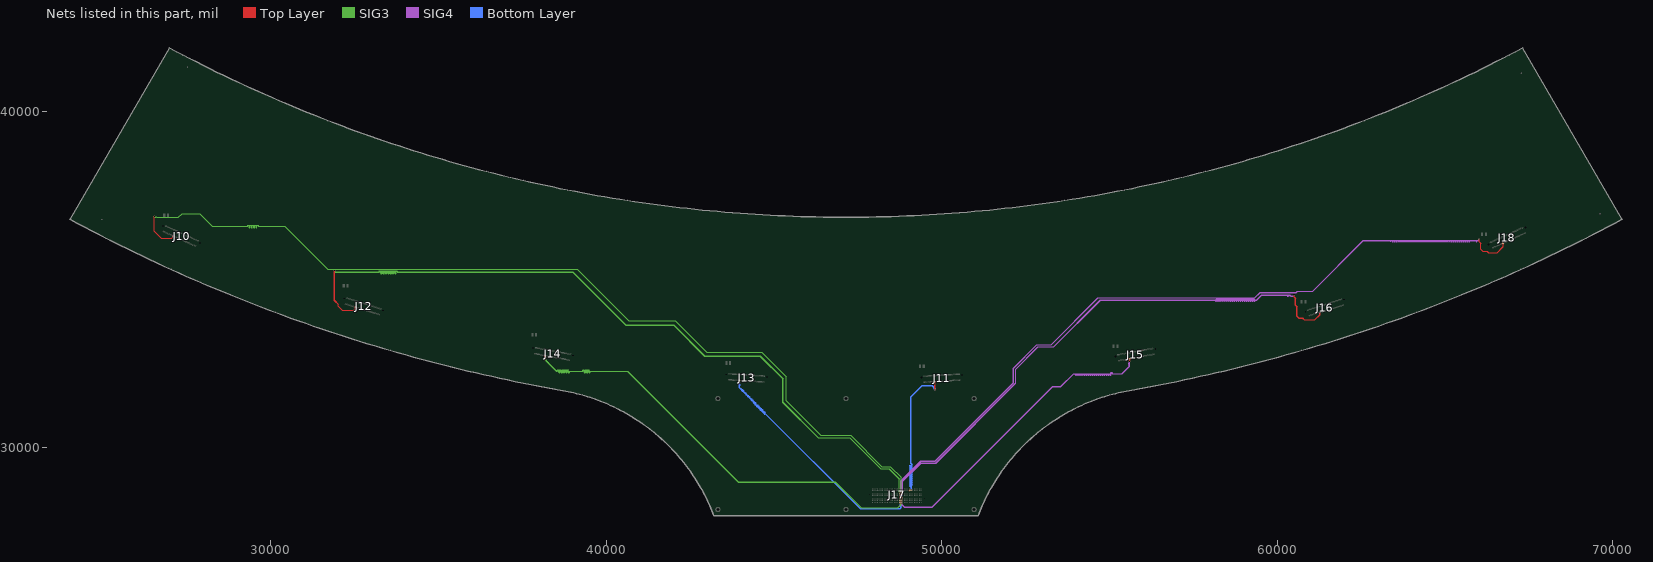
[diagram p0: the nets of this part, all layers, seen from the top]
# Altium PCB MISC86329.PcbDoc (part 5 of 11)
Units mil, origin at the board's own origin, x right, y up, seen from the top; angles counter-clockwise.
Board outline 46247.15 x 13937.21 mil, 6 copper layers (Top Layer, GND2, SIG3, SIG4, POWER5, Bottom Layer); 17 components, 210 nets, 908 pads, 1109 vias.

## Via types
v1: diameter 24, hole 12, Top Layer to Bottom Layer, 684 vias
v2: diameter 18, hole 9, Top Layer to Bottom Layer, 425 vias

## Nets (pads, with @x,y where several pads share a name; then routed paths per layer and width w, separated by ;. In a path a pad name is that pad's centre, name@x,y a point inside that pad or via, vN(x,y) a via of type N, cw(c..) or ccw(c..) an arc to the next point about the centre after c; other vN are vias at no path point) (continued)
DATAIN3N_CH1: J12.23 J17.F14 | length 23101.3
  Top Layer w5: v2(31893.5,35275) 31900,35268.5 31900,34381.86 32013,34268.86 32013,34213.86 32139.86,34087 32489.14,34087 32533.06,34130.92 32533.06,34159.09 J12.23@32553.09,34179.11 ; J17.F14@48737.89,28618.8 v2(48761.69,28642.61)
  SIG3 w5: v2(31893.5,35275) 31900,35268.5 31900,35252.86 31921.43,35231.43 ; 31920,35233 31929,35224 32003,35224 ; 31986.86,35224 32003,35224 ; v2(48761.69,28642.61) 48759.39,28642.61 48749.96,28652.04 48732,28670 48732,29060 48428,29364 48181.86,29364 47259.86,30286 46320.86,30286 45264,31342.86 45264,32047 44583,32728 42928.86,32728 42011.86,33645 40582.86,33645 39003.86,35224 33783.18,35224 33771.5,35235.68 33771.5,35257.84 33765.68,35263.67 33752.32,35263.67 33746.5,35257.84 33746.5,35196.01 33734.82,35184.33 33713.18,35184.33 33701.5,35196.01 33701.5,35257.84 33695.68,35263.67 33682.32,35263.67 33676.5,35257.84 33676.5,35196.01 33664.82,35184.33 33643.18,35184.33 33631.5,35196.01 33631.5,35257.84 33625.68,35263.67 33612.32,35263.67 33606.5,35257.84 33606.5,35196.01 33594.82,35184.33 33573.18,35184.33 33561.5,35196.01 33561.5,35257.84 33555.68,35263.67 33542.32,35263.67 33536.5,35257.84 33536.5,35196.01 33524.82,35184.33 33503.18,35184.33 33491.5,35196.01 33491.5,35257.84 33485.68,35263.67 33472.32,35263.67 33466.5,35257.84 33466.5,35196.01 33454.82,35184.33 33433.18,35184.33 33421.5,35196.01 33421.5,35257.84 33415.68,35263.67 33402.32,35263.67 33396.5,35257.84 33396.5,35196.01 33384.82,35184.33 33363.18,35184.33 33351.5,35196.01 33351.5,35257.84 33345.68,35263.67 33332.32,35263.67 33326.5,35257.84 33326.5,35196.01 33314.82,35184.33 33293.18,35184.33 33281.5,35196.01 33281.5,35257.84 33275.68,35263.67 33262.32,35263.67 33256.5,35257.84 33256.5,35235.68 33244.82,35224 32003,35224
DATAIN3N_CH2: J14.23 J17.B14 | length 13805.7
  Top Layer w5: v2(38195.5,32680) 38189,32686.5 38189,32711 38200,32722 J14.23@38200,32734 ; J17.B14@48737.89,28418.8 v2(48761.69,28395)
  SIG3 w5: v2@38194,32677 38188,32671 38188,32618 38192.42,32613.58 38201.26,32613.58 38202.28,32614.6 38211.11,32614.6 38219.95,32605.76 38219.95,32596.92 38218.94,32595.9 38218.94,32587.06 38227.77,32578.23 38236.61,32578.23 38237.56,32579.18 38246.4,32579.18 38255.24,32570.34 38255.24,32561.5 38254.29,32560.55 38254.29,32551.71 38263.13,32542.87 38271.97,32542.87 38272.92,32543.82 38281.76,32543.82 38290.6,32534.98 38290.6,32526.14 38289.65,32525.19 38289.65,32516.35 38526,32280 38546.68,32280 38552.5,32285.82 38552.5,32308.32 38564.18,32320 38585.82,32320 38597.5,32308.32 38597.5,32245.82 38603.32,32240 38616.68,32240 38622.5,32245.82 38622.5,32308.32 38634.18,32320 38655.82,32320 38667.5,32308.32 38667.5,32245.82 38673.32,32240 38686.68,32240 38692.5,32245.82 38692.5,32308.32 38704.18,32320 38725.82,32320 38737.5,32308.32 38737.5,32245.82 38743.32,32240 38756.68,32240 38762.5,32245.82 38762.5,32308.32 38774.18,32320 38795.82,32320 38807.5,32308.32 38807.5,32245.82 38813.32,32240 38826.68,32240 38832.5,32245.82 38832.5,32308.32 38844.18,32320 38865.82,32320 38877.5,32308.32 38877.5,32245.82 38883.32,32240 38896.68,32240 38902.5,32245.82 38902.5,32268.32 38914.18,32280 39302.68,32280 39308.5,32285.82 39308.5,32304.42 39320.18,32316.1 39341.82,32316.1 39353.5,32304.42 39353.5,32249.72 39359.32,32243.9 39372.68,32243.9 39378.5,32249.72 39378.5,32304.42 39390.18,32316.1 39411.82,32316.1 39423.5,32304.42 39423.5,32249.72 39429.32,32243.9 39442.68,32243.9 39448.5,32249.72 39448.5,32304.42 39460.18,32316.1 39481.82,32316.1 39493.5,32304.42 39493.5,32249.72 39499.32,32243.9 39512.68,32243.9 39518.5,32249.72 39518.5,32268.32 39530.18,32280 40641,32280 43937,28984 46829,28984 47603,28210 48693.69,28210 48781.69,28298 48781.69,28375 v2(48761.69,28395)
DATAIN3N_CH3: J13.23 J17.A14 | length 7749.3
  Top Layer w5: 43978.23,31941.5 43978.23,31959.28 43988.94,31970 J13.23@43988.94,31998.95 ; J17.A14@48737.89,28368.8 v2(48761.69,28345)
  Bottom Layer w5: v2(43984.73,31935) 43984.73,31934.67 43978,31927.94 43978,31893.5 43983,31888.5 43996.72,31888.5 44001.72,31883.5 44001.72,31868.5 43996.72,31863.5 43983,31863.5 43978,31858.5 43978,31783.14 43995.03,31766.12 43999.72,31766.12 44005.03,31771.42 44018.01,31771.42 44029.77,31759.65 44029.77,31746.67 44024.47,31741.37 44024.47,31736.67 44030.38,31730.76 44035.08,31730.76 44040.38,31736.06 44053.36,31736.06 44065.13,31724.3 44065.13,31711.32 44059.83,31706.01 44059.83,31701.32 44065.74,31695.41 44070.43,31695.41 44075.74,31700.71 44088.72,31700.71 44100.49,31688.94 44100.49,31675.96 44095.18,31670.66 44095.18,31665.96 44101.09,31660.05 44105.79,31660.05 44111.09,31665.35 44124.07,31665.35 44135.84,31653.59 44135.84,31640.6 44130.54,31635.3 44130.54,31630.6 44136.45,31624.69 44141.14,31624.69 44146.45,31630 44159.43,31630 44171.2,31618.23 44171.2,31605.25 44165.89,31599.95 44165.89,31595.25 44171.8,31589.34 44176.5,31589.34 44181.8,31594.64 44194.78,31594.64 44206.55,31582.88 44206.55,31569.89 44201.25,31564.59 44201.25,31559.89 44207.16,31553.98 44211.85,31553.98 44217.16,31559.29 44230.14,31559.29 44241.91,31547.52 44241.91,31534.54 44236.6,31529.24 44236.6,31524.54 44242.51,31518.63 44247.21,31518.63 44252.51,31523.93 44265.49,31523.93 44277.26,31512.16 44277.26,31499.18 44271.96,31493.88 44271.96,31489.18 44277.87,31483.27 44282.57,31483.27 44287.87,31488.58 44300.85,31488.58 44312.62,31476.81 44312.62,31463.83 44307.31,31458.52 44307.31,31453.83 44313.22,31447.92 44317.92,31447.92 44323.22,31453.22 44336.2,31453.22 44347.97,31441.45 44347.97,31428.47 44342.67,31423.17 44342.67,31418.47 44348.58,31412.56 44353.28,31412.56 44358.58,31417.87 44371.56,31417.87 44383.33,31406.1 44383.33,31393.12 44378.02,31387.81 44378.02,31383.12 44383.93,31377.21 44388.63,31377.21 44393.93,31382.51 44406.92,31382.51 44418.68,31370.74 44418.68,31357.76 44399.24,31338.32 44399.24,31333.62 44405.15,31327.71 44409.84,31327.71 44429.29,31347.16 44442.27,31347.16 44454.04,31335.39 44454.04,31322.41 44434.59,31302.96 44434.59,31298.26 44440.5,31292.35 44445.2,31292.35 44464.65,31311.8 44477.63,31311.8 44489.39,31300.03 44489.39,31287.05 44469.95,31267.61 44469.95,31262.91 44475.86,31257 44480.56,31257 44500,31276.44 44512.98,31276.44 44524.75,31264.68 44524.75,31251.7 44505.3,31232.25 44505.3,31227.55 44511.21,31221.64 44515.91,31221.64 44535.36,31241.09 44548.34,31241.09 44560.1,31229.32 44560.1,31216.34 44540.66,31196.9 44540.66,31192.2 44546.57,31186.29 44551.27,31186.29 44570.71,31205.73 44583.69,31205.73 44595.46,31193.97 44595.46,31180.99 44576.01,31161.54 44576.01,31156.84 44581.92,31150.93 44586.62,31150.93 44606.07,31170.38 44619.05,31170.38 44630.82,31158.61 44630.82,31145.63 44611.37,31126.18 44611.37,31121.49 44617.28,31115.58 44621.98,31115.58 44641.42,31135.02 44654.4,31135.02 44666.17,31123.26 44666.17,31110.27 44646.73,31090.83 44646.73,31086.13 44652.64,31080.22 44657.33,31080.22 44676.78,31099.67 44689.76,31099.67 44701.53,31087.9 44701.53,31074.92 44682.08,31055.47 44682.08,31050.78 44687.99,31044.87 44692.69,31044.87 44712.13,31064.31 44725.11,31064.31 44736.88,31052.54 44736.88,31039.56 44717.44,31020.12 44717.44,31015.42 44723.35,31009.51 44728.04,31009.51 44731.53,31013 44748.14,31013 47576.14,28185 48759,28185 48781.69,28207.69 48781.69,28223.18 48778.37,28226.5 48770.87,28226.5 48761.69,28235.68 48761.69,28252.32 48770.87,28261.5 48798.37,28261.5 48801.69,28264.82 48801.69,28273.18 48798.37,28276.5 48770.87,28276.5 48761.69,28285.68 48761.69,28302.32 48770.87,28311.5 48778.37,28311.5 48781.69,28314.82 48781.69,28325 v2(48761.69,28345)
DATAIN3N_CH4: J11.23 J17.H8 | length 5094.4
  Top Layer w5: J17.H8@49037.89,28718.8 v2(49061.69,28742.61) ; 49809.93,31719.5 49809.93,31933.28 49820.65,31944 J11.23@49820.65,31969.08
  Bottom Layer w5: v2(49061.69,28742.61) 49081.69,28762.61 49081.69,28831.93 49075.62,28838 49063.62,28838 49051.69,28849.93 49051.69,28866.07 49063.62,28878 49105.62,28878 49111.69,28884.07 49111.69,28891.93 49105.62,28898 49063.62,28898 49051.69,28909.93 49051.69,28926.07 49063.62,28938 49105.62,28938 49111.69,28944.07 49111.69,28951.93 49105.62,28958 49063.62,28958 49051.69,28969.93 49051.69,28986.07 49063.62,28998 49105.62,28998 49111.69,29004.07 49111.69,29011.93 49105.62,29018 49063.62,29018 49051.69,29029.93 49051.69,29046.07 49063.62,29058 49105.62,29058 49111.69,29064.07 49111.69,29071.93 49105.62,29078 49063.62,29078 49051.69,29089.93 49051.69,29106.07 49063.62,29118 49105.62,29118 49111.69,29124.07 49111.69,29131.93 49105.62,29138 49063.62,29138 49051.69,29149.93 49051.69,29166.07 49063.62,29178 49105.62,29178 49111.69,29184.07 49111.69,29191.93 49105.62,29198 49063.62,29198 49051.69,29209.93 49051.69,29226.07 49063.62,29238 49105.62,29238 49111.69,29244.07 49111.69,29251.93 49105.62,29258 49063.62,29258 49051.69,29269.93 49051.69,29286.07 49063.62,29298 49105.62,29298 49111.69,29304.07 49111.69,29311.93 49105.62,29318 49063.62,29318 49051.69,29329.93 49051.69,29346.07 49063.62,29358 49105.62,29358 49111.69,29364.07 49111.69,29371.93 49105.62,29378 49063.62,29378 49051.69,29389.93 49051.69,29406.07 49063.62,29418 49105.62,29418 49111.69,29424.07 49111.69,29431.93 49105.62,29438 49063.62,29438 49051.69,29449.93 49051.69,29466.07 49063.62,29478 49101.86,29478 49108,29484.14 49108,29496 49081.69,29522.31 49081.69,31519.69 49421,31859 49712.14,31859 49810,31761.14 49810,31720 v2@49814,31716
  other v2: 49816.43,31713
DATAIN3N_CH5: J15.23 J17.C14 | length 10126
  Top Layer w5: J17.C14@48737.89,28468.8 v2(48761.69,28445) ; v2(55610.5,32567) 55604,32573.5 55604,32615.47 55612.53,32624 J15.23@55612.53,32650.14
  SIG4 w5: v2(48761.69,28445) 48781.69,28425 48781.69,28323.17 48878.86,28226 49724.14,28226 53312.14,31814 53553,31814 53936,32197 53981.43,32197 53986,32192.43 53986,32169.16 53996.43,32158.73 54015.57,32158.73 54026,32169.16 54026,32192.43 54030.57,32197 54041.43,32197 54046,32192.43 54046,32169.16 54056.43,32158.73 54075.57,32158.73 54086,32169.16 54086,32192.43 54090.57,32197 54101.43,32197 54106,32192.43 54106,32169.16 54116.43,32158.73 54135.57,32158.73 54146,32169.16 54146,32192.43 54150.57,32197 54161.43,32197 54166,32192.43 54166,32169.16 54176.43,32158.73 54195.57,32158.73 54206,32169.16 54206,32192.43 54210.57,32197 54221.43,32197 54226,32192.43 54226,32169.16 54236.43,32158.73 54255.57,32158.73 54266,32169.16 54266,32192.43 54270.57,32197 54281.43,32197 54286,32192.43 54286,32169.16 54296.43,32158.73 54315.57,32158.73 54326,32169.16 54326,32192.43 54330.57,32197 54341.43,32197 54346,32192.43 54346,32169.16 54356.43,32158.73 54375.57,32158.73 54386,32169.16 54386,32192.43 54390.57,32197 54401.43,32197 54406,32192.43 54406,32169.16 54416.43,32158.73 54435.57,32158.73 54446,32169.16 54446,32192.43 54450.57,32197 54461.43,32197 54466,32192.43 54466,32169.16 54476.43,32158.73 54495.57,32158.73 54506,32169.16 54506,32192.43 54510.57,32197 54521.43,32197 54526,32192.43 54526,32169.16 54536.43,32158.73 54555.57,32158.73 54566,32169.16 54566,32192.43 54570.57,32197 54581.43,32197 54586,32192.43 54586,32169.16 54596.43,32158.73 54615.57,32158.73 54626,32169.16 54626,32192.43 54630.57,32197 54641.43,32197 54646,32192.43 54646,32169.16 54656.43,32158.73 54675.57,32158.73 54686,32169.16 54686,32192.43 54690.57,32197 54701.43,32197 54706,32192.43 54706,32169.16 54716.43,32158.73 54735.57,32158.73 54746,32169.16 54746,32192.43 54750.57,32197 54761.43,32197 54766,32192.43 54766,32169.16 54776.43,32158.73 54795.57,32158.73 54806,32169.16 54806,32192.43 54810.57,32197 54821.43,32197 54826,32192.43 54826,32169.16 54836.43,32158.73 54855.57,32158.73 54866,32169.16 54866,32192.43 54870.57,32197 54881.43,32197 54886,32192.43 54886,32169.16 54896.43,32158.73 54915.57,32158.73 54926,32169.16 54926,32192.43 54930.57,32197 54941.43,32197 54946,32192.43 54946,32169.16 54956.43,32158.73 54975.57,32158.73 54986,32169.16 54986,32192.43 54990.57,32197 55001.43,32197 55006,32192.43 55006,32169.16 55016.43,32158.73 55035.57,32158.73 55046,32169.16 55046,32230.69 55050.57,32235.27 55061.43,32235.27 55066,32230.69 55066,32207.43 55076.43,32197 55377,32197 55604,32424 55604,32441 55604,32447 55604,32477 55604,32487 55604,32517 55604,32532 55604,32542 55604,32558 v2@55610,32564
DATAIN3N_CH6: J16.23 J17.D14 | length 18293.9
  Top Layer w5: J17.D14@48737.89,28518.8 v2(48761.69,28495) ; v2(60484.5,34554) 60491,34547.5 60491,34491 60535,34447 60535,34235 60581,34189 60581,33910.86 60635.86,33856 60747.86,33856 60800.86,33803 61119.14,33803 61277,33960.86 61277,34003.76 61278.24,34005 J16.23@61278.24,34031.97
  SIG4 w5: v2(48761.69,28495) 48788.36,28495 48804.86,28511.5 48814.05,28511.5 48830,28527.45 48830,28997.14 49382.86,29550 49827,29550 52202,31925 52202,32341.14 52867.86,33007 53336,33007 54730,34401 58144,34401 58167.93,34377.07 58168,34377.07 58172.07,34373 58181.86,34373 58188,34379.14 58188,34419.07 58199.93,34431 58216.07,34431 58228,34419.07 58228,34377.07 58234.07,34371 58241.93,34371 58248,34377.07 58248,34419.07 58259.93,34431 58276.07,34431 58288,34419.07 58288,34377.07 58294.07,34371 58301.93,34371 58308,34377.07 58308,34419.07 58319.93,34431 58336.07,34431 58348,34419.07 58348,34377.07 58354.07,34371 58361.93,34371 58368,34377.07 58368,34419.07 58379.93,34431 58396.07,34431 58408,34419.07 58408,34377.07 58414.07,34371 58421.93,34371 58428,34377.07 58428,34419.07 58439.93,34431 58456.07,34431 58468,34419.07 58468,34377.07 58474.07,34371 58481.93,34371 58488,34377.07 58488,34419.07 58499.93,34431 58516.07,34431 58528,34419.07 58528,34377.07 58534.07,34371 58541.93,34371 58548,34377.07 58548,34419.07 58559.93,34431 58576.07,34431 58588,34419.07 58588,34377.07 58594.07,34371 58601.93,34371 58608,34377.07 58608,34419.07 58619.93,34431 58636.07,34431 58648,34419.07 58648,34377.07 58654.07,34371 58661.93,34371 58668,34377.07 58668,34419.07 58679.93,34431 58696.07,34431 58708,34419.07 58708,34377.07 58714.07,34371 58721.93,34371 58728,34377.07 58728,34419.07 58739.93,34431 58756.07,34431 58768,34419.07 58768,34377.07 58774.07,34371 58781.93,34371 58788,34377.07 58788,34419.07 58799.93,34431 58816.07,34431 58828,34419.07 58828,34377.07 58834.07,34371 58841.93,34371 58848,34377.07 58848,34419.07 58859.93,34431 58876.07,34431 58888,34419.07 58888,34377.07 58894.07,34371 58901.93,34371 58908,34377.07 58908,34419.07 58919.93,34431 58936.07,34431 58948,34419.07 58948,34377.07 58954.07,34371 58961.93,34371 58968,34377.07 58968,34419.07 58979.93,34431 58996.07,34431 59008,34419.07 59008,34377.07 59014.07,34371 59021.93,34371 59028,34377.07 59028,34419.07 59039.93,34431 59056.07,34431 59068,34419.07 59068,34377.07 59074.07,34371 59081.93,34371 59088,34377.07 59088,34419.07 59099.93,34431 59116.07,34431 59128,34419.07 59128,34377.07 59134.07,34371 59141.93,34371 59148,34377.07 59148,34419.07 59159.93,34431 59176.07,34431 59188,34419.07 59188,34377.07 59194.07,34371 59201.93,34371 59208,34377.07 59208,34419.07 59219.93,34431 59236.07,34431 59248,34419.07 59248,34377.07 59254.07,34371 59261.93,34371 59268,34377.07 59268,34419.07 59279.93,34431 59296.07,34431 59308,34419.07 59308,34377.07 59314.07,34371 59321.93,34371 59328,34377.07 59328,34389.07 59339.93,34401 59383,34401 59531,34549 60378.14,34549 60404.14,34523 60479,34523 60491,34535 60491,34546 v2@60485,34552
DATAIN3N_CH7: J17.E14 J18.23 | length 23897.1
  Top Layer w5: J17.E14@48737.89,28568.8 v2(48761.69,28545) ; v2(66004.5,36214) 66011,36207.5 66011,36128 66059,36080 66059,35901.86 66115.86,35845 66246.86,35845 66289.86,35802 66551.14,35802 66737,35987.86 66737,36062.73 66733.02,36066.71 66733.31,36067 J18.23@66733.31,36093.98
  SIG4 w5: v2(48761.69,28545) 48781.69,28565 48781.69,29010.83 49379.86,29609 49804,29609 52132,31937 52132,32370.14 52832.86,33071 53261,33071 54657,34467 59331,34467 59488,34624 60560,34624 60601,34665 61050,34665 62563,36178 63346,36178 63369,36155 63378.86,36155 63401.86,36178 63421.07,36178 63431.5,36167.57 63431.5,36152.57 63436.07,36148 63446.93,36148 63451.5,36152.57 63451.5,36167.57 63461.93,36178 63481.07,36178 63491.5,36167.57 63491.5,36152.57 63496.07,36148 63506.93,36148 63511.5,36152.57 63511.5,36167.57 63521.93,36178 63541.07,36178 63551.5,36167.57 63551.5,36152.57 63556.07,36148 63566.93,36148 63571.5,36152.57 63571.5,36167.57 63581.93,36178 63601.07,36178 63611.5,36167.57 63611.5,36152.57 63616.07,36148 63626.93,36148 63631.5,36152.57 63631.5,36167.57 63641.93,36178 63661.07,36178 63671.5,36167.57 63671.5,36152.57 63676.07,36148 63686.93,36148 63691.5,36152.57 63691.5,36167.57 63701.93,36178 63721.07,36178 63731.5,36167.57 63731.5,36152.57 63736.07,36148 63746.93,36148 63751.5,36152.57 63751.5,36167.57 63761.93,36178 63781.07,36178 63791.5,36167.57 63791.5,36152.57 63796.07,36148 63806.93,36148 63811.5,36152.57 63811.5,36167.57 63821.93,36178 63841.07,36178 63851.5,36167.57 63851.5,36152.57 63856.07,36148 63866.93,36148 63871.5,36152.57 63871.5,36167.57 63881.93,36178 63901.07,36178 63911.5,36167.57 63911.5,36152.57 63916.07,36148 63926.93,36148 63931.5,36152.57 63931.5,36167.57 63941.93,36178 63961.07,36178 63971.5,36167.57 63971.5,36152.57 63976.07,36148 63986.93,36148 63991.5,36152.57 63991.5,36167.57 64001.93,36178 64021.07,36178 64031.5,36167.57 64031.5,36152.57 64036.07,36148 64046.93,36148 64051.5,36152.57 64051.5,36167.57 64061.93,36178 64081.07,36178 64091.5,36167.57 64091.5,36152.57 64096.07,36148 64106.93,36148 64111.5,36152.57 64111.5,36167.57 64121.93,36178 64141.07,36178 64151.5,36167.57 64151.5,36152.57 64156.07,36148 64166.93,36148 64171.5,36152.57 64171.5,36167.57 64181.93,36178 64201.07,36178 64211.5,36167.57 64211.5,36152.57 64216.07,36148 64226.93,36148 64231.5,36152.57 64231.5,36167.57 64241.93,36178 64261.07,36178 64271.5,36167.57 64271.5,36152.57 64276.07,36148 64286.93,36148 64291.5,36152.57 64291.5,36167.57 64301.93,36178 64321.07,36178 64331.5,36167.57 64331.5,36152.57 64336.07,36148 64346.93,36148 64351.5,36152.57 64351.5,36167.57 64361.93,36178 64381.07,36178 64391.5,36167.57 64391.5,36152.57 64396.07,36148 64406.93,36148 64411.5,36152.57 64411.5,36167.57 64421.93,36178 64441.07,36178 64451.5,36167.57 64451.5,36152.57 64456.07,36148 64466.93,36148 64471.5,36152.57 64471.5,36167.57 64481.93,36178 64501.07,36178 64511.5,36167.57 64511.5,36152.57 64516.07,36148 64526.93,36148 64531.5,36152.57 64531.5,36167.57 64541.93,36178 64561.07,36178 64571.5,36167.57 64571.5,36152.57 64576.07,36148 64586.93,36148 64591.5,36152.57 64591.5,36167.57 64601.93,36178 64621.07,36178 64631.5,36167.57 64631.5,36152.57 64636.07,36148 64646.93,36148 64651.5,36152.57 64651.5,36167.57 64661.93,36178 64681.07,36178 64691.5,36167.57 64691.5,36152.57 64696.07,36148 64706.93,36148 64711.5,36152.57 64711.5,36167.57 64721.93,36178 64741.07,36178 64751.5,36167.57 64751.5,36152.57 64756.07,36148 64766.93,36148 64771.5,36152.57 64771.5,36167.57 64781.93,36178 64801.07,36178 64811.5,36167.57 64811.5,36152.57 64816.07,36148 64826.93,36148 64831.5,36152.57 64831.5,36167.57 64841.93,36178 64861.07,36178 64871.5,36167.57 64871.5,36152.57 64876.07,36148 64886.93,36148 64891.5,36152.57 64891.5,36167.57 64901.93,36178 64921.07,36178 64931.5,36167.57 64931.5,36152.57 64936.07,36148 64946.93,36148 64951.5,36152.57 64951.5,36167.57 64961.93,36178 64981.07,36178 64991.5,36167.57 64991.5,36152.57 64996.07,36148 65006.93,36148 65011.5,36152.57 65011.5,36167.57 65021.93,36178 65041.07,36178 65051.5,36167.57 65051.5,36152.57 65056.07,36148 65066.93,36148 65071.5,36152.57 65071.5,36167.57 65081.93,36178 65101.07,36178 65111.5,36167.57 65111.5,36152.57 65116.07,36148 65126.93,36148 65131.5,36152.57 65131.5,36167.57 65141.93,36178 65161.07,36178 65171.5,36167.57 65171.5,36152.57 65176.07,36148 65186.93,36148 65191.5,36152.57 65191.5,36167.57 65201.93,36178 65221.07,36178 65231.5,36167.57 65231.5,36152.57 65236.07,36148 65246.93,36148 65251.5,36152.57 65251.5,36167.57 65261.93,36178 65281.07,36178 65291.5,36167.57 65291.5,36152.57 65296.07,36148 65306.93,36148 65311.5,36152.57 65311.5,36167.57 65321.93,36178 65341.07,36178 65351.5,36167.57 65351.5,36152.57 65356.07,36148 65366.93,36148 65371.5,36152.57 65371.5,36167.57 65381.93,36178 65401.07,36178 65411.5,36167.57 65411.5,36152.57 65416.07,36148 65426.93,36148 65431.5,36152.57 65431.5,36167.57 65441.93,36178 65461.07,36178 65471.5,36167.57 65471.5,36152.57 65476.07,36148 65486.93,36148 65491.5,36152.57 65491.5,36167.57 65501.93,36178 65521.07,36178 65531.5,36167.57 65531.5,36152.57 65536.07,36148 65546.93,36148 65551.5,36152.57 65551.5,36167.57 65561.93,36178 65581.07,36178 65591.5,36167.57 65591.5,36152.57 65596.07,36148 65606.93,36148 65611.5,36152.57 65611.5,36167.57 65621.93,36178 65641.07,36178 65651.5,36167.57 65651.5,36152.57 65656.07,36148 65666.93,36148 65671.5,36152.57 65671.5,36167.57 65681.93,36178 65701.07,36178 65711.5,36167.57 65711.5,36152.57 65716.07,36148 65726.93,36148 65731.5,36152.57 65731.5,36167.57 65741.93,36178 65988.86,36178 66011,36200.14 66011,36206 v2@66004,36213
DATAIN3P_CH0: J10.21 J17.G13 | length 28226.7
  Top Layer w5: v2(26545.5,36894) 26539,36887.5 26539,36452 26747,36244 27066,36244 27090.78,36268.78 J10.21@27090.78,36309.99 ; J17.G13@48787.89,28668.8 v2(48811.69,28692.61)
  SIG3 w5: v2(26545.5,36894) 26539,36887.5 26539,36872 26549,36862 26580,36862 26585,36867 26585,36876.47 26590,36881.47 26600,36881.47 26605,36876.47 26605,36867 26610,36862 27256.86,36862 27364.86,36970 27891,36970 28272,36589 29311.68,36589 29317.5,36594.82 29317.5,36616.56 29329.18,36628.24 29350.82,36628.24 29362.5,36616.56 29362.5,36555.59 29368.32,36549.76 29381.68,36549.76 29387.5,36555.59 29387.5,36616.56 29399.18,36628.24 29420.82,36628.24 29432.5,36616.56 29432.5,36555.59 29438.32,36549.76 29451.68,36549.76 29457.5,36555.59 29457.5,36616.56 29469.18,36628.24 29490.82,36628.24 29502.5,36616.56 29502.5,36555.59 29508.32,36549.76 29521.68,36549.76 29527.5,36555.59 29527.5,36616.56 29539.18,36628.24 29560.82,36628.24 29572.5,36616.56 29572.5,36555.59 29578.32,36549.76 29591.68,36549.76 29597.5,36555.59 29597.5,36616.56 29609.18,36628.24 29630.82,36628.24 29642.5,36616.56 29642.5,36594.82 29648.32,36589 30433,36589 31713,35309 39136,35309 40672,33773 42063,33773 42999,32837 44638.14,32837 45362,32113.14 45362,31394 46392,30364 47288,30364 48219,29433 48467.14,29433 48791.69,29108.45 48791.69,28712.61 v2(48811.69,28692.61)
DATAIN3P_CH1: J12.21 J17.F13 | length 23088.7
  Top Layer w5: v2(31916.5,35275) 31910,35268.5 31910,34386 32023,34273 32023,34218 32144,34097 32485,34097 32523.06,34135.06 J12.21@32523.06,34188.62 ; J17.F13@48787.89,28618.8 v2(48811.69,28642.61)
  SIG3 w5: v2(31916.5,35275) 31910,35268.5 31910,35257 31924,35243 31924.14,35243 31933.14,35234 32003,35234 33240.68,35234 33246.5,35239.82 33246.5,35261.99 33258.18,35273.67 33279.82,35273.67 33291.5,35261.99 33291.5,35200.16 33297.32,35194.33 33310.68,35194.33 33316.5,35200.16 33316.5,35261.99 33328.18,35273.67 33349.82,35273.67 33361.5,35261.99 33361.5,35200.16 33367.32,35194.33 33380.68,35194.33 33386.5,35200.16 33386.5,35261.99 33398.18,35273.67 33419.82,35273.67 33431.5,35261.99 33431.5,35200.16 33437.32,35194.33 33450.68,35194.33 33456.5,35200.16 33456.5,35261.99 33468.18,35273.67 33489.82,35273.67 33501.5,35261.99 33501.5,35200.16 33507.32,35194.33 33520.68,35194.33 33526.5,35200.16 33526.5,35261.99 33538.18,35273.67 33559.82,35273.67 33571.5,35261.99 33571.5,35200.16 33577.32,35194.33 33590.68,35194.33 33596.5,35200.16 33596.5,35261.99 33608.18,35273.67 33629.82,35273.67 33641.5,35261.99 33641.5,35200.16 33647.32,35194.33 33660.68,35194.33 33666.5,35200.16 33666.5,35261.99 33678.18,35273.67 33699.82,35273.67 33711.5,35261.99 33711.5,35200.16 33717.32,35194.33 33730.68,35194.33 33736.5,35200.16 33736.5,35261.99 33748.18,35273.67 33769.82,35273.67 33781.5,35261.99 33781.5,35239.82 33787.32,35234 39008,35234 40587,33655 42016,33655 42933,32738 44587.14,32738 45274,32051.14 45274,31347 46325,30296 47264,30296 48186,29374 48432.14,29374 48742,29064.14 48742,28674.14 48757.04,28659.11 48768.53,28659.11 48785.03,28642.61 v2(48811.69,28642.61)
DATAIN3P_CH2: J14.21 J17.B13 | length 13806.3
  Top Layer w5: J14.21@38173.38,32745.09 38173.38,32719 38179,32713.38 38179,32686.5 ; J17.B13@48787.89,28418.8 v2(48811.69,28395)
  SIG3 w5: v2(38172.5,32680) v2@38179,32680 ; v2@38173,32678 38178,32673 38178,32613.86 38521.86,32270 38550.82,32270 38562.5,32281.68 38562.5,32304.18 38568.32,32310 38581.68,32310 38587.5,32304.18 38587.5,32241.68 38599.18,32230 38620.82,32230 38632.5,32241.68 38632.5,32304.18 38638.32,32310 38651.68,32310 38657.5,32304.18 38657.5,32241.68 38669.18,32230 38690.82,32230 38702.5,32241.68 38702.5,32304.18 38708.32,32310 38721.68,32310 38727.5,32304.18 38727.5,32241.68 38739.18,32230 38760.82,32230 38772.5,32241.68 38772.5,32304.18 38778.32,32310 38791.68,32310 38797.5,32304.18 38797.5,32241.68 38809.18,32230 38830.82,32230 38842.5,32241.68 38842.5,32304.18 38848.32,32310 38861.68,32310 38867.5,32304.18 38867.5,32241.68 38879.18,32230 38900.82,32230 38912.5,32241.68 38912.5,32264.18 38918.32,32270 39306.82,32270 39318.5,32281.68 39318.5,32300.28 39324.32,32306.1 39337.68,32306.1 39343.5,32300.28 39343.5,32245.58 39355.18,32233.9 39376.82,32233.9 39388.5,32245.58 39388.5,32300.28 39394.32,32306.1 39407.68,32306.1 39413.5,32300.28 39413.5,32245.58 39425.18,32233.9 39446.82,32233.9 39458.5,32245.58 39458.5,32300.28 39464.32,32306.1 39477.68,32306.1 39483.5,32300.28 39483.5,32245.58 39495.18,32233.9 39516.82,32233.9 39528.5,32245.58 39528.5,32264.18 39534.32,32270 40636.86,32270 43932.86,28974 46824.86,28974 47598.86,28200 48697.83,28200 48791.69,28293.86 48791.69,28375 v2(48811.69,28395)
DATAIN3P_CH3: J13.21 J17.A13 | length 7749.7
  Top Layer w5: J13.21@43957.51,32000.91 43957.51,31975 43968.23,31964.28 43968.23,31941.5 ; J17.A13@48787.89,28368.8 v2(48811.69,28345)
  Bottom Layer w5: v2@43964,31934 43963,31935 43963,31933 43968,31928 43968,31914.25 ; 43968,31914.55 43968,31914.25 ; v2(48811.69,28345) 48791.69,28325 48791.69,28310.68 48782.51,28301.5 48775.01,28301.5 48771.69,28298.18 48771.69,28289.82 48775.01,28286.5 48802.51,28286.5 48811.69,28277.32 48811.69,28260.68 48802.51,28251.5 48775.01,28251.5 48771.69,28248.18 48771.69,28239.82 48775.01,28236.5 48782.51,28236.5 48791.69,28227.32 48791.69,28203.55 48763.14,28175 47572,28175 44744,31003 44735.67,31003 44732.18,30999.51 44719.2,30999.51 44707.44,31011.28 44707.44,31024.26 44726.88,31043.71 44726.88,31048.4 44720.97,31054.31 44716.27,31054.31 44696.83,31034.87 44683.85,31034.87 44672.08,31046.63 44672.08,31059.62 44691.53,31079.06 44691.53,31083.76 44685.62,31089.67 44680.92,31089.67 44661.47,31070.22 44648.49,31070.22 44636.73,31081.99 44636.73,31094.97 44656.17,31114.42 44656.17,31119.11 44650.26,31125.02 44645.56,31125.02 44626.12,31105.58 44613.14,31105.58 44601.37,31117.35 44601.37,31130.33 44620.82,31149.77 44620.82,31154.47 44614.91,31160.38 44610.21,31160.38 44590.76,31140.93 44577.78,31140.93 44566.01,31152.7 44566.01,31165.68 44585.46,31185.13 44585.46,31189.82 44579.55,31195.73 44574.85,31195.73 44555.41,31176.29 44542.43,31176.29 44530.66,31188.06 44530.66,31201.04 44550.1,31220.48 44550.1,31225.18 44544.19,31231.09 44539.5,31231.09 44520.05,31211.64 44507.07,31211.64 44495.3,31223.41 44495.3,31236.39 44514.75,31255.84 44514.75,31260.53 44508.84,31266.44 44504.14,31266.44 44484.7,31247 44471.72,31247 44459.95,31258.77 44459.95,31271.75 44479.39,31291.19 44479.39,31295.89 44473.48,31301.8 44468.79,31301.8 44449.34,31282.35 44436.36,31282.35 44424.59,31294.12 44424.59,31307.1 44444.04,31326.55 44444.04,31331.25 44438.13,31337.16 44433.43,31337.16 44413.99,31317.71 44401.01,31317.71 44389.24,31329.48 44389.24,31342.46 44408.68,31361.9 44408.68,31366.6 44402.77,31372.51 44398.08,31372.51 44392.77,31367.21 44379.79,31367.21 44368.02,31378.98 44368.02,31391.96 44373.33,31397.26 44373.33,31401.96 44367.42,31407.87 44362.72,31407.87 44357.42,31402.56 44344.44,31402.56 44332.67,31414.33 44332.67,31427.31 44337.97,31432.61 44337.97,31437.31 44332.06,31443.22 44327.37,31443.22 44322.06,31437.92 44309.08,31437.92 44297.31,31449.69 44297.31,31462.67 44302.62,31467.97 44302.62,31472.67 44296.71,31478.58 44292.01,31478.58 44286.71,31473.27 44273.73,31473.27 44261.96,31485.04 44261.96,31498.02 44267.26,31503.33 44267.26,31508.02 44261.35,31513.93 44256.66,31513.93 44251.35,31508.63 44238.37,31508.63 44226.6,31520.4 44226.6,31533.38 44231.91,31538.68 44231.91,31543.38 44226,31549.29 44221.3,31549.29 44216,31543.98 44203.02,31543.98 44191.25,31555.75 44191.25,31568.73 44196.55,31574.04 44196.55,31578.73 44190.64,31584.64 44185.94,31584.64 44180.64,31579.34 44167.66,31579.34 44155.89,31591.11 44155.89,31604.09 44161.2,31609.39 44161.2,31614.09 44155.29,31620 44150.59,31620 44145.29,31614.69 44132.31,31614.69 44120.54,31626.46 44120.54,31639.44 44125.84,31644.75 44125.84,31649.44 44119.93,31655.35 44115.23,31655.35 44109.93,31650.05 44096.95,31650.05 44085.18,31661.82 44085.18,31674.8 44090.49,31680.1 44090.49,31684.8 44084.58,31690.71 44079.88,31690.71 44074.58,31685.41 44061.59,31685.41 44049.83,31697.17 44049.83,31710.15 44055.13,31715.46 44055.13,31720.15 44049.22,31726.06 44044.52,31726.06 44039.22,31720.76 44026.24,31720.76 44014.47,31732.53 44014.47,31745.51 44019.77,31750.81 44019.77,31755.51 44013.86,31761.42 44009.17,31761.42 44003.86,31756.12 43990.88,31756.12 43968,31779 43968,31914.25
  other v2: 43961.73,31935
DATAIN3P_CH4: J11.21 J17.H7 | length 5094.2
  Top Layer w5: J17.H7@49087.89,28718.8 v2(49111.69,28742.61) ; J11.21@49789.21,31967.2 49789.21,31942 49799.93,31931.28 49799.93,31719.5
  Bottom Layer w5: v2(49111.69,28742.61) 49091.69,28762.61 49091.69,28836.07 49079.76,28848 49067.76,28848 49061.69,28854.07 49061.69,28861.93 49067.76,28868 49109.76,28868 49121.69,28879.93 49121.69,28896.07 49109.76,28908 49067.76,28908 49061.69,28914.07 49061.69,28921.93 49067.76,28928 49109.76,28928 49121.69,28939.93 49121.69,28956.07 49109.76,28968 49067.76,28968 49061.69,28974.07 49061.69,28981.93 49067.76,28988 49109.76,28988 49121.69,28999.93 49121.69,29016.07 49109.76,29028 49067.76,29028 49061.69,29034.07 49061.69,29041.93 49067.76,29048 49109.76,29048 49121.69,29059.93 49121.69,29076.07 49109.76,29088 49067.76,29088 49061.69,29094.07 49061.69,29101.93 49067.76,29108 49109.76,29108 49121.69,29119.93 49121.69,29136.07 49109.76,29148 49067.76,29148 49061.69,29154.07 49061.69,29161.93 49067.76,29168 49109.76,29168 49121.69,29179.93 49121.69,29196.07 49109.76,29208 49067.76,29208 49061.69,29214.07 49061.69,29221.93 49067.76,29228 49109.76,29228 49121.69,29239.93 49121.69,29256.07 49109.76,29268 49067.76,29268 49061.69,29274.07 49061.69,29281.93 49067.76,29288 49109.76,29288 49121.69,29299.93 49121.69,29316.07 49109.76,29328 49067.76,29328 49061.69,29334.07 49061.69,29341.93 49067.76,29348 49109.76,29348 49121.69,29359.93 49121.69,29376.07 49109.76,29388 49067.76,29388 49061.69,29394.07 49061.69,29401.93 49067.76,29408 49109.76,29408 49121.69,29419.93 49121.69,29436.07 49109.76,29448 49067.76,29448 49061.69,29454.07 49061.69,29461.93 49067.76,29468 49106,29468 49118,29480 49118,29500.14 49091.69,29526.45 49091.69,31515.55 49425.14,31849 49708,31849 49768.75,31788.25 49768.75,31781.18 49760.38,31772.81 49760.38,31765.74 49767.45,31758.67 49774.53,31758.67 49782.89,31767.04 49789.96,31767.04 49800,31757 49800,31720 v2@49794,31714
  other v2: 49793.43,31713
DATAIN3P_CH5: J15.21 J17.C13 | length 10126
  Top Layer w5: J17.C13@48787.89,28468.8 v2(48811.69,28445) ; J15.21@55581.56,32644.44 55581.56,32618 55594,32605.56 55594,32573.5
  SIG4 w5: v2(48811.69,28445) 48791.69,28425 48791.69,28327.31 48883,28236 49720,28236 53308,31824 53548.86,31824 53931.86,32207 53985.57,32207 53996,32196.57 53996,32173.31 54000.57,32168.73 54011.43,32168.73 54016,32173.31 54016,32196.57 54026.43,32207 54045.57,32207 54056,32196.57 54056,32173.31 54060.57,32168.73 54071.43,32168.73 54076,32173.31 54076,32196.57 54086.43,32207 54105.57,32207 54116,32196.57 54116,32173.31 54120.57,32168.73 54131.43,32168.73 54136,32173.31 54136,32196.57 54146.43,32207 54165.57,32207 54176,32196.57 54176,32173.31 54180.57,32168.73 54191.43,32168.73 54196,32173.31 54196,32196.57 54206.43,32207 54225.57,32207 54236,32196.57 54236,32173.31 54240.57,32168.73 54251.43,32168.73 54256,32173.31 54256,32196.57 54266.43,32207 54285.57,32207 54296,32196.57 54296,32173.31 54300.57,32168.73 54311.43,32168.73 54316,32173.31 54316,32196.57 54326.43,32207 54345.57,32207 54356,32196.57 54356,32173.31 54360.57,32168.73 54371.43,32168.73 54376,32173.31 54376,32196.57 54386.43,32207 54405.57,32207 54416,32196.57 54416,32173.31 54420.57,32168.73 54431.43,32168.73 54436,32173.31 54436,32196.57 54446.43,32207 54465.57,32207 54476,32196.57 54476,32173.31 54480.57,32168.73 54491.43,32168.73 54496,32173.31 54496,32196.57 54506.43,32207 54525.57,32207 54536,32196.57 54536,32173.31 54540.57,32168.73 54551.43,32168.73 54556,32173.31 54556,32196.57 54566.43,32207 54585.57,32207 54596,32196.57 54596,32173.31 54600.57,32168.73 54611.43,32168.73 54616,32173.31 54616,32196.57 54626.43,32207 54645.57,32207 54656,32196.57 54656,32173.31 54660.57,32168.73 54671.43,32168.73 54676,32173.31 54676,32196.57 54686.43,32207 54705.57,32207 54716,32196.57 54716,32173.31 54720.57,32168.73 54731.43,32168.73 54736,32173.31 54736,32196.57 54746.43,32207 54765.57,32207 54776,32196.57 54776,32173.31 54780.57,32168.73 54791.43,32168.73 54796,32173.31 54796,32196.57 54806.43,32207 54825.57,32207 54836,32196.57 54836,32173.31 54840.57,32168.73 54851.43,32168.73 54856,32173.31 54856,32196.57 54866.43,32207 54885.57,32207 54896,32196.57 54896,32173.31 54900.57,32168.73 54911.43,32168.73 54916,32173.31 54916,32196.57 54926.43,32207 54945.57,32207 54956,32196.57 54956,32173.31 54960.57,32168.73 54971.43,32168.73 54976,32173.31 54976,32196.57 54986.43,32207 55005.57,32207 55016,32196.57 55016,32173.31 55020.57,32168.73 55031.43,32168.73 55036,32173.31 55036,32234.84 55046.43,32245.27 55065.57,32245.27 55076,32234.84 55076,32211.57 55080.57,32207 55372.86,32207 55594,32428.14 55594,32441 55594,32447 55589,32452 55581.6,32452 55576.6,32457 55576.6,32467 55581.6,32472 55589,32472 55594,32477 55594,32487 55589,32492 55581.6,32492 55576.6,32497 55576.6,32507 55581.6,32512 55589,32512 55594,32517 55594,32532 55594,32542 55594,32561 v2@55590,32565
  other v2: 55587.5,32567
DATAIN3P_CH6: J16.21 J17.D13 | length 18293.3
  Top Layer w5: J17.D13@48787.89,28518.8 v2(48811.69,28495) ; v2(60507.5,34554) 60501,34547.5 60501,34495.14 60545,34451.14 60545,34239.14 60591,34193.14 60591,33915 60640,33866 60752,33866 60805,33813 61115,33813 61267,33965 61267,34003.73 J16.21@61248.19,34022.54
  SIG4 w5: v2(48811.69,28495) 48840,28523.31 48840,28993 49387,29540 49831.14,29540 52212,31920.86 52212,32337 52872,32997 53340.14,32997 54734.14,34391 58139.86,34391 58167.86,34363 58186,34363 58198,34375 58198,34414.93 58204.07,34421 58211.93,34421 58218,34414.93 58218,34372.93 58229.93,34361 58246.07,34361 58258,34372.93 58258,34414.93 58264.07,34421 58271.93,34421 58278,34414.93 58278,34372.93 58289.93,34361 58306.07,34361 58318,34372.93 58318,34414.93 58324.07,34421 58331.93,34421 58338,34414.93 58338,34372.93 58349.93,34361 58366.07,34361 58378,34372.93 58378,34414.93 58384.07,34421 58391.93,34421 58398,34414.93 58398,34372.93 58409.93,34361 58426.07,34361 58438,34372.93 58438,34414.93 58444.07,34421 58451.93,34421 58458,34414.93 58458,34372.93 58469.93,34361 58486.07,34361 58498,34372.93 58498,34414.93 58504.07,34421 58511.93,34421 58518,34414.93 58518,34372.93 58529.93,34361 58546.07,34361 58558,34372.93 58558,34414.93 58564.07,34421 58571.93,34421 58578,34414.93 58578,34372.93 58589.93,34361 58606.07,34361 58618,34372.93 58618,34414.93 58624.07,34421 58631.93,34421 58638,34414.93 58638,34372.93 58649.93,34361 58666.07,34361 58678,34372.93 58678,34414.93 58684.07,34421 58691.93,34421 58698,34414.93 58698,34372.93 58709.93,34361 58726.07,34361 58738,34372.93 58738,34414.93 58744.07,34421 58751.93,34421 58758,34414.93 58758,34372.93 58769.93,34361 58786.07,34361 58798,34372.93 58798,34414.93 58804.07,34421 58811.93,34421 58818,34414.93 58818,34372.93 58829.93,34361 58846.07,34361 58858,34372.93 58858,34414.93 58864.07,34421 58871.93,34421 58878,34414.93 58878,34372.93 58889.93,34361 58906.07,34361 58918,34372.93 58918,34414.93 58924.07,34421 58931.93,34421 58938,34414.93 58938,34372.93 58949.93,34361 58966.07,34361 58978,34372.93 58978,34414.93 58984.07,34421 58991.93,34421 58998,34414.93 58998,34372.93 59009.93,34361 59026.07,34361 59038,34372.93 59038,34414.93 59044.07,34421 59051.93,34421 59058,34414.93 59058,34372.93 59069.93,34361 59086.07,34361 59098,34372.93 59098,34414.93 59104.07,34421 59111.93,34421 59118,34414.93 59118,34372.93 59129.93,34361 59146.07,34361 59158,34372.93 59158,34414.93 59164.07,34421 59171.93,34421 59178,34414.93 59178,34372.93 59189.93,34361 59206.07,34361 59218,34372.93 59218,34414.93 59224.07,34421 59231.93,34421 59238,34414.93 59238,34372.93 59249.93,34361 59266.07,34361 59278,34372.93 59278,34414.93 59284.07,34421 59291.93,34421 59298,34414.93 59298,34372.93 59309.93,34361 59326.07,34361 59338,34372.93 59338,34384.93 59344.07,34391 59387.14,34391 59535.14,34539 60285,34539 60290,34534 60290,34520.06 60295,34515.06 60305,34515.06 60310,34520.06 60310,34534 60315,34539 60325,34539 60330,34534 60330,34520.06 60335,34515.06 60345,34515.06 60350,34520.06 60350,34534 60355,34539 60374,34539 60400,34513 60483.14,34513 60501,34530.86 60501,34546 v2@60507,34552
DATAIN3P_CH7: J17.E13 J18.21 | length 23896.7
  Top Layer w5: J17.E13@48787.89,28568.8 v2(48811.69,28545) ; v2(66027.5,36214) 66021,36207.5 66021,36132.14 66069,36084.14 66069,35906 66120,35855 66251,35855 66294,35812 66547,35812 66727,35992 66727,36058.59 J18.21@66704.64,36080.95
  SIG4 w5: v2(48811.69,28545) 48791.69,28565 48791.69,29006.69 49384,29599 49808.14,29599 52142,31932.86 52142,32366 52837,33061 53265.14,33061 54661.14,34457 59335.14,34457 59492.14,34614 60564.14,34614 60605.14,34655 61054.14,34655 62567.14,36168 63341.86,36168 63364.86,36145 63383,36145 63401.43,36163.43 63401.5,36163.43 63406.07,36168 63416.93,36168 63421.5,36163.43 63421.5,36148.43 63431.93,36138 63451.07,36138 63461.5,36148.43 63461.5,36163.43 63466.07,36168 63476.93,36168 63481.5,36163.43 63481.5,36148.43 63491.93,36138 63511.07,36138 63521.5,36148.43 63521.5,36163.43 63526.07,36168 63536.93,36168 63541.5,36163.43 63541.5,36148.43 63551.93,36138 63571.07,36138 63581.5,36148.43 63581.5,36163.43 63586.07,36168 63596.93,36168 63601.5,36163.43 63601.5,36148.43 63611.93,36138 63631.07,36138 63641.5,36148.43 63641.5,36163.43 63646.07,36168 63656.93,36168 63661.5,36163.43 63661.5,36148.43 63671.93,36138 63691.07,36138 63701.5,36148.43 63701.5,36163.43 63706.07,36168 63716.93,36168 63721.5,36163.43 63721.5,36148.43 63731.93,36138 63751.07,36138 63761.5,36148.43 63761.5,36163.43 63766.07,36168 63776.93,36168 63781.5,36163.43 63781.5,36148.43 63791.93,36138 63811.07,36138 63821.5,36148.43 63821.5,36163.43 63826.07,36168 63836.93,36168 63841.5,36163.43 63841.5,36148.43 63851.93,36138 63871.07,36138 63881.5,36148.43 63881.5,36163.43 63886.07,36168 63896.93,36168 63901.5,36163.43 63901.5,36148.43 63911.93,36138 63931.07,36138 63941.5,36148.43 63941.5,36163.43 63946.07,36168 63956.93,36168 63961.5,36163.43 63961.5,36148.43 63971.93,36138 63991.07,36138 64001.5,36148.43 64001.5,36163.43 64006.07,36168 64016.93,36168 64021.5,36163.43 64021.5,36148.43 64031.93,36138 64051.07,36138 64061.5,36148.43 64061.5,36163.43 64066.07,36168 64076.93,36168 64081.5,36163.43 64081.5,36148.43 64091.93,36138 64111.07,36138 64121.5,36148.43 64121.5,36163.43 64126.07,36168 64136.93,36168 64141.5,36163.43 64141.5,36148.43 64151.93,36138 64171.07,36138 64181.5,36148.43 64181.5,36163.43 64186.07,36168 64196.93,36168 64201.5,36163.43 64201.5,36148.43 64211.93,36138 64231.07,36138 64241.5,36148.43 64241.5,36163.43 64246.07,36168 64256.93,36168 64261.5,36163.43 64261.5,36148.43 64271.93,36138 64291.07,36138 64301.5,36148.43 64301.5,36163.43 64306.07,36168 64316.93,36168 64321.5,36163.43 64321.5,36148.43 64331.93,36138 64351.07,36138 64361.5,36148.43 64361.5,36163.43 64366.07,36168 64376.93,36168 64381.5,36163.43 64381.5,36148.43 64391.93,36138 64411.07,36138 64421.5,36148.43 64421.5,36163.43 64426.07,36168 64436.93,36168 64441.5,36163.43 64441.5,36148.43 64451.93,36138 64471.07,36138 64481.5,36148.43 64481.5,36163.43 64486.07,36168 64496.93,36168 64501.5,36163.43 64501.5,36148.43 64511.93,36138 64531.07,36138 64541.5,36148.43 64541.5,36163.43 64546.07,36168 64556.93,36168 64561.5,36163.43 64561.5,36148.43 64571.93,36138 64591.07,36138 64601.5,36148.43 64601.5,36163.43 64606.07,36168 64616.93,36168 64621.5,36163.43 64621.5,36148.43 64631.93,36138 64651.07,36138 64661.5,36148.43 64661.5,36163.43 64666.07,36168 64676.93,36168 64681.5,36163.43 64681.5,36148.43 64691.93,36138 64711.07,36138 64721.5,36148.43 64721.5,36163.43 64726.07,36168 64736.93,36168 64741.5,36163.43 64741.5,36148.43 64751.93,36138 64771.07,36138 64781.5,36148.43 64781.5,36163.43 64786.07,36168 64796.93,36168 64801.5,36163.43 64801.5,36148.43 64811.93,36138 64831.07,36138 64841.5,36148.43 64841.5,36163.43 64846.07,36168 64856.93,36168 64861.5,36163.43 64861.5,36148.43 64871.93,36138 64891.07,36138 64901.5,36148.43 64901.5,36163.43 64906.07,36168 64916.93,36168 64921.5,36163.43 64921.5,36148.43 64931.93,36138 64951.07,36138 64961.5,36148.43 64961.5,36163.43 64966.07,36168 64976.93,36168 64981.5,36163.43 64981.5,36148.43 64991.93,36138 65011.07,36138 65021.5,36148.43 65021.5,36163.43 65026.07,36168 65036.93,36168 65041.5,36163.43 65041.5,36148.43 65051.93,36138 65071.07,36138 65081.5,36148.43 65081.5,36163.43 65086.07,36168 65096.93,36168 65101.5,36163.43 65101.5,36148.43 65111.93,36138 65131.07,36138 65141.5,36148.43 65141.5,36163.43 65146.07,36168 65156.93,36168 65161.5,36163.43 65161.5,36148.43 65171.93,36138 65191.07,36138 65201.5,36148.43 65201.5,36163.43 65206.07,36168 65216.93,36168 65221.5,36163.43 65221.5,36148.43 65231.93,36138 65251.07,36138 65261.5,36148.43 65261.5,36163.43 65266.07,36168 65276.93,36168 65281.5,36163.43 65281.5,36148.43 65291.93,36138 65311.07,36138 65321.5,36148.43 65321.5,36163.43 65326.07,36168 65336.93,36168 65341.5,36163.43 65341.5,36148.43 65351.93,36138 65371.07,36138 65381.5,36148.43 65381.5,36163.43 65386.07,36168 65396.93,36168 65401.5,36163.43 65401.5,36148.43 65411.93,36138 65431.07,36138 65441.5,36148.43 65441.5,36163.43 65446.07,36168 65456.93,36168 65461.5,36163.43 65461.5,36148.43 65471.93,36138 65491.07,36138 65501.5,36148.43 65501.5,36163.43 65506.07,36168 65516.93,36168 65521.5,36163.43 65521.5,36148.43 65531.93,36138 65551.07,36138 65561.5,36148.43 65561.5,36163.43 65566.07,36168 65576.93,36168 65581.5,36163.43 65581.5,36148.43 65591.93,36138 65611.07,36138 65621.5,36148.43 65621.5,36163.43 65626.07,36168 65636.93,36168 65641.5,36163.43 65641.5,36148.43 65651.93,36138 65671.07,36138 65681.5,36148.43 65681.5,36163.43 65686.07,36168 65696.93,36168 65701.5,36163.43 65701.5,36148.43 65711.93,36138 65731.07,36138 65741.5,36148.43 65741.5,36163.43 65746.07,36168 65917,36168 65922,36163 65922,36143.83 65927,36138.83 65937,36138.83 65942,36143.83 65942,36163 65947,36168 65993,36168 66021,36196 66021,36207.5